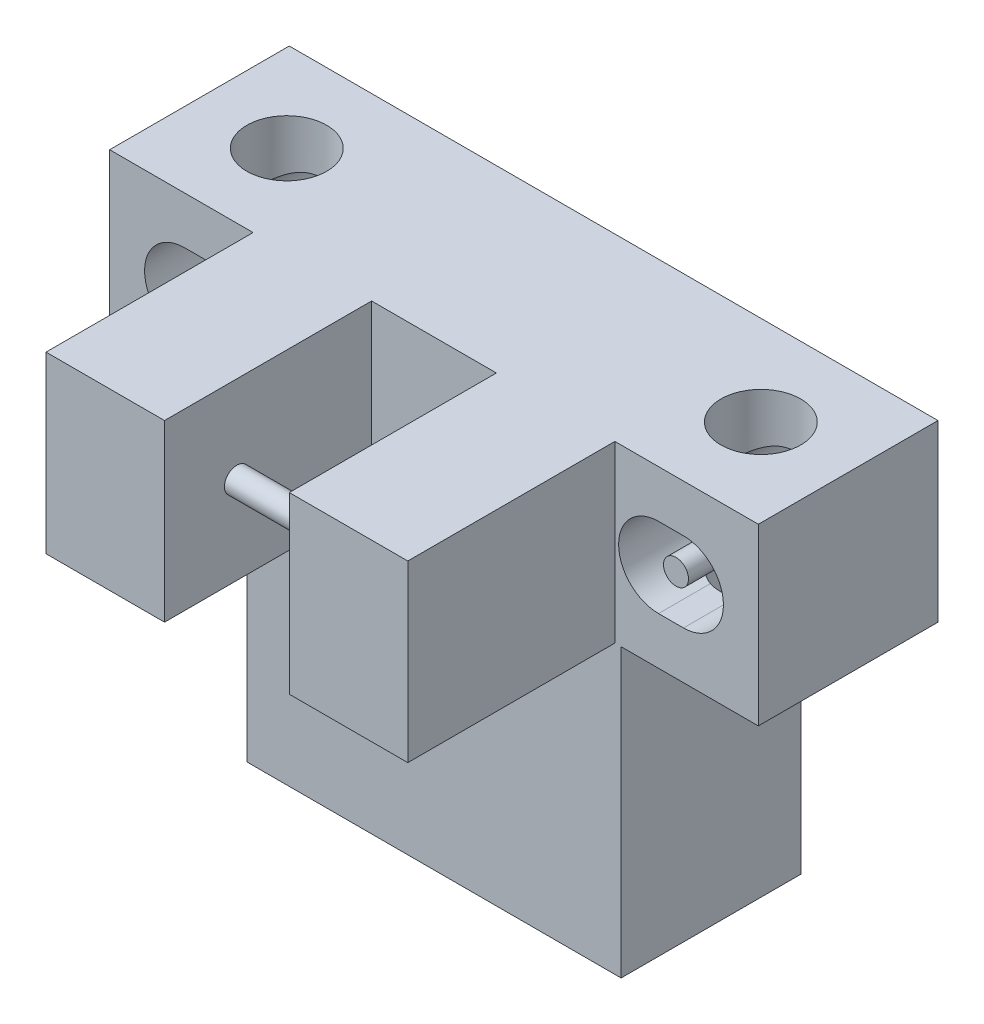
SolidWorks part; units mm, degrees
material "6061 合金"
ref_plane "前视基准面" through (0, 0, 0) normal (0, 0, 1) x (1, 0, 0)
ref_plane "上视基准面" through (0, 0, 0) normal (0, 1, 0) x (1, 0, 0)
ref_plane "右视基准面" through (0, 0, 0) normal (1, 0, 0) x (0, 0, -1)
sketch "草图1" plane through (0, 0, 0) normal (0, 0, 1) x (1, 0, 0)
  line L0 (0, 0) -> (0, 18.5) construction
  line L1 (13, 18.5) -> (-13, 18.5)
  line L2 (-13, 18.5) -> (-13, 11.5)
  line L3 (-13, 11.5) -> (-7.5, 11.5)
  line L4 (-7.5, 11.5) -> (-7.5, 0)
  line L5 (-7.5, 0) -> (7.5, 0)
  line L6 (7.5, 11.5) -> (7.5, 0)
  line L7 (13, 11.5) -> (7.5, 11.5)
  line L8 (13, 18.5) -> (13, 11.5)
  line L9 (-10, 15) -> (-9, 15) construction
  line L10 (-10, 16.6) -> (-9, 16.6)
  line L11 (-10, 13.4) -> (-9, 13.4)
  line L12 (-13, 15) -> (13, 15) construction
  line L13 (10, 15) -> (9, 15) construction
  line L14 (10, 16.6) -> (9, 16.6)
  line L15 (10, 13.4) -> (9, 13.4)
  arc A0 (-10, 16.6) -> (-10, 13.4) centre (-10, 15) ccw
  arc A1 (-9, 13.4) -> (-9, 16.6) centre (-9, 15) ccw
  arc A2 (10, 16.6) -> (10, 13.4) centre (10, 15) cw
  arc A3 (9, 13.4) -> (9, 16.6) centre (9, 15) cw
  point P13 (-9.5, 15)
  point P22 (9.5, 15)
  dimension "D5" = 1.6
  dimension "D1" = 26
  dimension "D2" = 7
  dimension "D3" = 18.5
  dimension "D4" = 15
  dimension "D6" = 1
  dimension "D7" = 19
extrude "凸台-拉伸1" add sketch "草图1" along normal mid plane 7.2
sketch "草图2" plane through (0, 0, 3.6) normal (0, 0, 1) x (1, 0, 0)
  line L0 (0, 18.5) -> (0, 0) construction
  line L1 (13, 18.5) -> (-13, 18.5) construction
  line L2 (-13, 11.5) -> (-7.5, 11.5) construction
  line L3 (-2.5, 18.5) -> (-7.25, 18.5)
  line L4 (-2.5, 18.5) -> (-2.5, 11.5)
  line L5 (-2.5, 11.5) -> (-7.25, 11.5)
  line L6 (-7.25, 18.5) -> (-7.25, 11.5)
  line L7 (7.25, 18.5) -> (7.25, 11.5)
  line L8 (2.5, 11.5) -> (7.25, 11.5)
  line L9 (2.5, 18.5) -> (2.5, 11.5)
  line L10 (2.5, 18.5) -> (7.25, 18.5)
  dimension "D1" = 5
  dimension "D2" = 14.5
extrude "凸台-拉伸2" add sketch "草图2" along normal offset from surface (8.3 mm away) 15.5 up to face at (-9.5, 15, -3.6)
sketch "草图3" plane through (-2.5, 0, 0) normal (1, 0, 0) x (0, 0, -1)
  line L0 (-11.9, 15) -> (-9, 15) construction
  line L1 (-11.9, 11.5) -> (-11.9, 18.5) construction
  circle A0 centre (-9, 15) radius 0.5
  dimension "D1" = 1
  dimension "D2" = 2.9
extrude "凸台-拉伸3" add sketch "草图3" along normal blind 9
hole_wizard "Ø3.2 (3.2) 直径孔1" positions "草图6" profile "草图5" hole size "Ø3.2" standard "GB" end condition through all
sketch "草图6" plane through (0, 18.5, 0) normal (0, 1, 0) x (1, 0, 0)
  line L0 (-9.5, 0) -> (9.5, 0) construction
  line L3 (0, 3.6) -> (0, 0) construction
  line L4 (13, 3.6) -> (-13, 3.6) construction
  point P0 (-9.5, 0)
  point P2 (9.5, 0)
  dimension "D1" = 19
  dimension "D2" = 3.6
sketch "草图5" plane through (-9.5, 18.5, 0) normal (1, 0, 0) x (0, 0, 1)
  line L0 (0, 0) -> (0, 18.5)
  line L1 (0, 18.5) -> (1.6, 18.5)
  line L2 (1.6, 18.5) -> (1.6, 0)
  line L5 (1.6, 0) -> (0, 0)
  line L11 (0, -6.35) -> (0, 107.95) construction
  dimension "通孔孔直径" = 3.2
  dimension "通孔孔深度" = 18.5
sketch "草图4" plane through (0, 0, -3.6) normal (0, 0, -1) x (-1, 0, 0)
  line L0 (11.6, 15) -> (7.4, 15) construction
  line L1 (0, 18.5) -> (0, 14.5) construction
  line L2 (-2.5, 18.5) -> (2.5, 18.5) construction
  line L3 (-2.5, 14.5) -> (2.5, 14.5) construction
  arc A0 (10, 13.4) -> (10, 16.6) centre (10, 15) ccw construction
  arc A1 (9, 16.6) -> (9, 13.4) centre (9, 15) ccw construction
  circle A2 centre (9.5, 15) radius 0.5
  circle A3 centre (-9.5, 15) radius 0.5
  dimension "D1" = 1
  dimension "D2" = 9.5
extrude "凸台-拉伸4" add sketch "草图4" against normal blind 7 separate body
